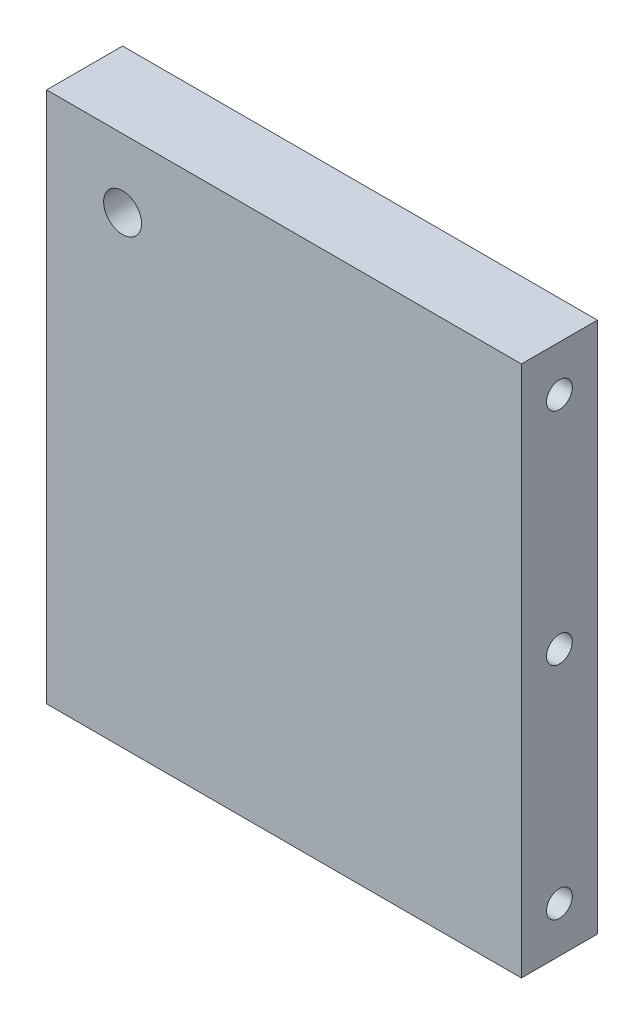
SolidWorks part; units mm, degrees
ref_plane "Front Plane" through (0, 0, 0) normal (0, 0, 1) x (1, 0, 0)
ref_plane "Top Plane" through (0, 0, 0) normal (0, 1, 0) x (1, 0, 0)
ref_plane "Right Plane" through (0, 0, 0) normal (1, 0, 0) x (0, 0, -1)
sketch "Sketch1" plane through (0, 0, 0) normal (0, 0, 1) x (1, 0, 0)
  line L1 (-62.5, 70) -> (62.5, 70)
  line L2 (-62.5, 70) -> (-62.5, -70)
  line L3 (-62.5, -70) -> (62.5, -70)
  line L4 (62.5, 70) -> (62.5, -70)
  line L5 (-62.5, 70) -> (62.5, -70) construction
  line L6 (-62.5, -70) -> (62.5, 70) construction
  point P0 (0, 0)
  dimension "D1" = 125
  dimension "D2" = 140
extrude "Boss-Extrude1" add sketch "Sketch1" along normal blind 20
hole_wizard "M10 Tapped Hole1" positions "Sketch3" profile "Sketch2" tap size "M10" standard "Iso"
sketch "Sketch3" plane through (-62.5, 0, 0) normal (-1, 0, 0) x (0, 0, 1)
  point P9 (10, 40)
  point P12 (10, 0)
  point P15 (10, -40)
sketch "Sketch2" plane through (-62.5, 40, 10) normal (0, 1, 0) x (0, 0, 1)
  line L0 (0, 0) -> (0, 37.5537)
  line L1 (0, 37.5537) -> (4.25, 35)
  line L2 (4.25, 35) -> (4.25, 0)
  line L5 (4.25, 0) -> (0, 0)
  line L10 (0, 37.5537) -> (-4.25, 35) construction
  line L11 (0, -6.35) -> (0, 107.95) construction
  dimension "螺纹孔钻头直径" = 8.5
  dimension "螺纹孔钻头深度" = 35
  dimension "导头角度" = 118
cosmetic thread "Cosmetic Thread4"
cosmetic thread "Cosmetic Thread5"
cosmetic thread "Cosmetic Thread6"
hole_wizard "M8 Tapped Hole1" positions "Sketch5" profile "Sketch4" tap size "M8" standard "Iso"
sketch "Sketch5" plane through (62.5, 0, 0) normal (1, 0, 0) x (0, 0, -1)
  point P0 (-10, 58)
  point P3 (-10, 0)
  point P6 (-10, -58)
sketch "Sketch4" plane through (62.5, 58, 10) normal (0, 1, 0) x (0, 0, -1)
  line L0 (0, 0) -> (0, 24.2929)
  line L1 (0, 24.2929) -> (3.4, 22.25)
  line L2 (3.4, 22.25) -> (3.4, 0)
  line L5 (3.4, 0) -> (0, 0)
  line L10 (0, 24.2929) -> (-3.4, 22.25) construction
  line L11 (0, -6.35) -> (0, 107.95) construction
  dimension "螺纹孔钻头直径" = 6.8
  dimension "螺纹孔钻头深度" = 22.25
  dimension "导头角度" = 118
cosmetic thread "Cosmetic Thread7"
cosmetic thread "Cosmetic Thread8"
cosmetic thread "Cosmetic Thread9"
sketch "Sketch6" plane through (0, 0, 20) normal (0, 0, 1) x (1, 0, 0)
  line L1 (-62.5, 70) -> (-62.5, -70) construction
  line L2 (62.5, 70) -> (-62.5, 70) construction
  circle A0 centre (-42.5, 52) radius 5
  dimension "D1" = 10
  dimension "D2" = 18
  dimension "D3" = 20
extrude "Cut-Extrude1" cut sketch "Sketch6" against normal through all
